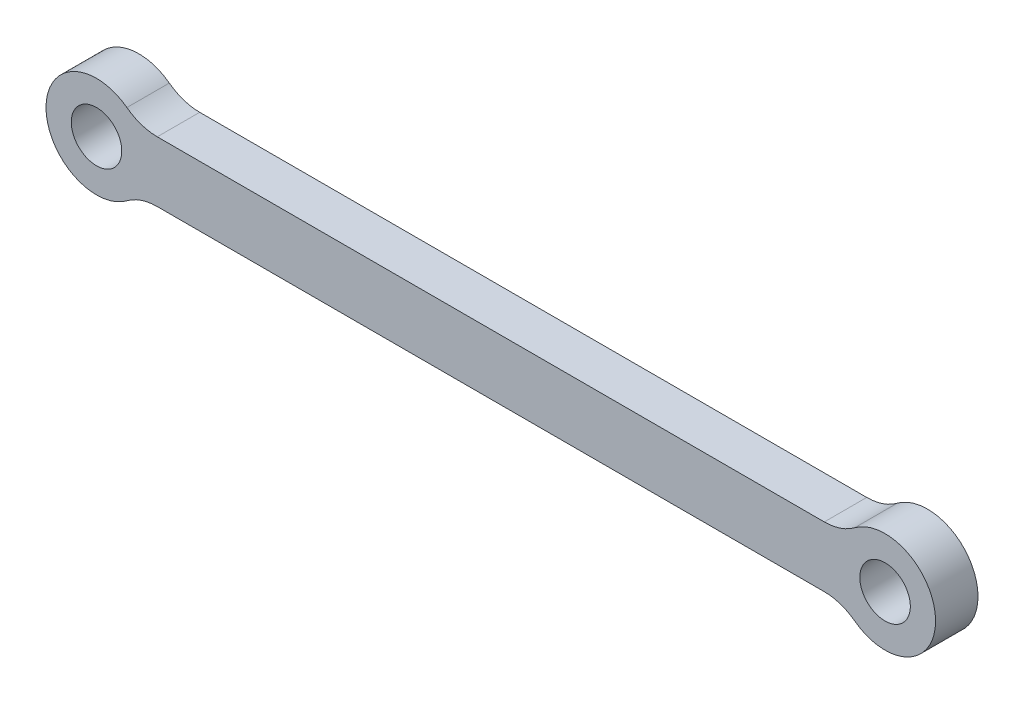
SolidWorks part; units mm, degrees
ref_plane "Front Plane" through (0, 0, 0) normal (0, 0, 1) x (1, 0, 0)
ref_plane "Top Plane" through (0, 0, 0) normal (0, 1, 0) x (1, 0, 0)
ref_plane "Right Plane" through (0, 0, 0) normal (1, 0, 0) x (0, 0, -1)
sketch "Sketch1" plane through (0, 0, 0) normal (0, 0, 1) x (1, 0, 0)
  line L0 (-737.5804, 0) -> (823.4196, 0)
  line L1 (-617.3265, 59.8092) -> (703.1656, 59.8092)
  line L2 (-617.3265, -59.8092) -> (703.1656, -59.8092)
  circle A0 centre (-737.5804, 0) radius 50
  arc A1 (-677.4535, 79.9046) -> (-677.4535, -79.9046) centre (-737.5804, 0) ccw
  circle A2 centre (823.4196, 0) radius 50
  arc A3 (763.2926, -79.9046) -> (763.2926, 79.9046) centre (823.4196, 0) ccw
  arc A4 (763.2926, -79.9046) -> (703.1656, -59.8092) centre (703.1656, -159.8092) ccw
  arc A5 (703.1656, 59.8092) -> (763.2926, 79.9046) centre (703.1656, 159.8092) ccw
  arc A6 (-617.3265, -59.8092) -> (-677.4535, -79.9046) centre (-617.3265, -159.8092) ccw
  arc A7 (-617.3265, 59.8092) -> (-677.4535, 79.9046) centre (-617.3265, 159.8092) cw
  point P11 (743.2768, -59.8092)
  point P14 (743.2768, 59.8092)
  point P17 (-657.4377, -59.8092)
  point P20 (-657.4377, 59.8092)
  dimension "D2" = 100
  dimension "D3" = 200
  dimension "D4" = 100
  dimension "D1" = 1561
sketch "Sketch2" plane through (0, 0, 0) normal (0, 0, 1) x (1, 0, 0)
extrude "Boss-Extrude1" add sketch "Sketch1" along normal blind 84
